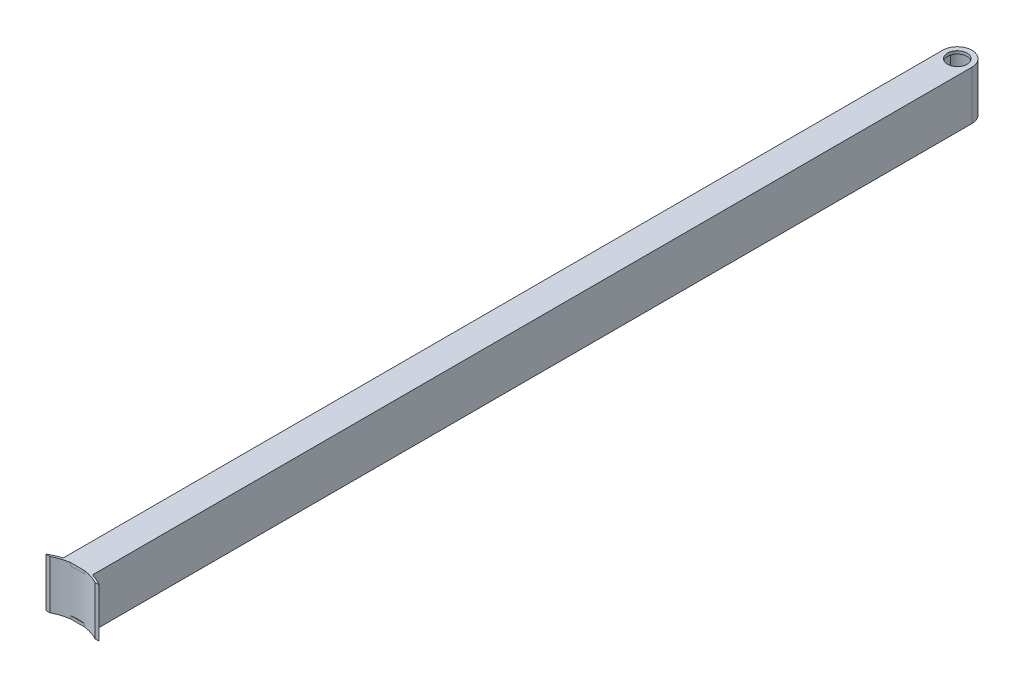
from build123d import *

# Parameters (mm, degrees)
SKETCH_1_W          = 30
SKETCH_1_H          = 50
SKETCH_1_W_2        = 24
SKETCH_1_H_2        = 44
EXTRUDE_1_DEPTH     = 900
SKETCH_2_R          = 10
CUT_EXTRUDE_2_DEPTH = 900
EXTRUDE_2_DEPTH     = 50
SKETCH_4_W          = 30
SKETCH_4_H          = 50
SKETCH_4_W_2        = 24
SKETCH_4_H_2        = 44
EXTRUDE_3_DEPTH     = 15
EXTRUDE_4_DEPTH     = 50


with BuildPart() as part:
    # 草图1 → 凸台-拉伸1 (new body)
    with BuildSketch(Plane.XY):
        with Locations((15, 25)):
            Rectangle(SKETCH_1_W, SKETCH_1_H)
        with Locations((15, 25)):
            Rectangle(SKETCH_1_W_2, SKETCH_1_H_2, mode=Mode.SUBTRACT)
    extrude(amount=EXTRUDE_1_DEPTH)

    # 草图2 → 切除-拉伸2 (cut)
    with BuildSketch(Plane(origin=(0, 50, 0), x_dir=(1, 0, 0), z_dir=(0, 1, 0))):
        with Locations(Location((15, -15, 0), (0, 0, 270))):
            Circle(SKETCH_2_R)
        with BuildLine():
            ThreePointArc((0, -15), (4.393398282, -4.393398282), (15, 0))
            Line((15, 0), (0, 0))
            Line((0, 0), (0, -15))
        make_face()
        with BuildLine():
            Line((30, 0), (15, 0))
            ThreePointArc((15, 0), (25.606601718, -4.393398282), (30, -15))
            Line((30, -15), (30, 0))
        make_face()
    extrude(amount=-CUT_EXTRUDE_2_DEPTH, mode=Mode.SUBTRACT)

    # 草图3 → 凸台-拉伸2 (add)
    with BuildSketch(Plane(origin=(0, 50, 0), x_dir=(1, 0, 0), z_dir=(0, 1, 0))):
        with BuildLine():
            Line((2, -15), (0, -15))
            ThreePointArc((0, -15), (15, 0), (30, -15))
            Line((30, -15), (28, -15))
            ThreePointArc((28, -15), (15, -2), (2, -15))
        make_face()
    extrude(amount=-EXTRUDE_2_DEPTH)

    # 草图4 → 凸台-拉伸3 (add)
    with BuildSketch(Plane.XY.offset(900)):
        with Locations((15, 25)):
            Rectangle(SKETCH_4_W, SKETCH_4_H)
        with Locations((15, 25)):
            Rectangle(SKETCH_4_W_2, SKETCH_4_H_2, mode=Mode.SUBTRACT)
    extrude(amount=EXTRUDE_3_DEPTH)

    # 草图5 → 凸台-拉伸4 (add)
    with BuildSketch(Plane(origin=(0, 50, 0), x_dir=(1, 0, 0), z_dir=(0, 1, 0))):
        with BuildLine():
            Line((-12.2207709, -920.098671199), (-8.128726759, -920.098671199))
            ThreePointArc((-8.128726759, -920.098671199), (15, -914.491908276), (38.128726759, -920.098671199))
            Line((38.128726759, -920.098671199), (42.2207709, -920.098671199))
            ThreePointArc((42.2207709, -920.098671199), (15, -912.491908276), (-12.2207709, -920.098671199))
        make_face()
    extrude(amount=-EXTRUDE_4_DEPTH)


solid = part.part
